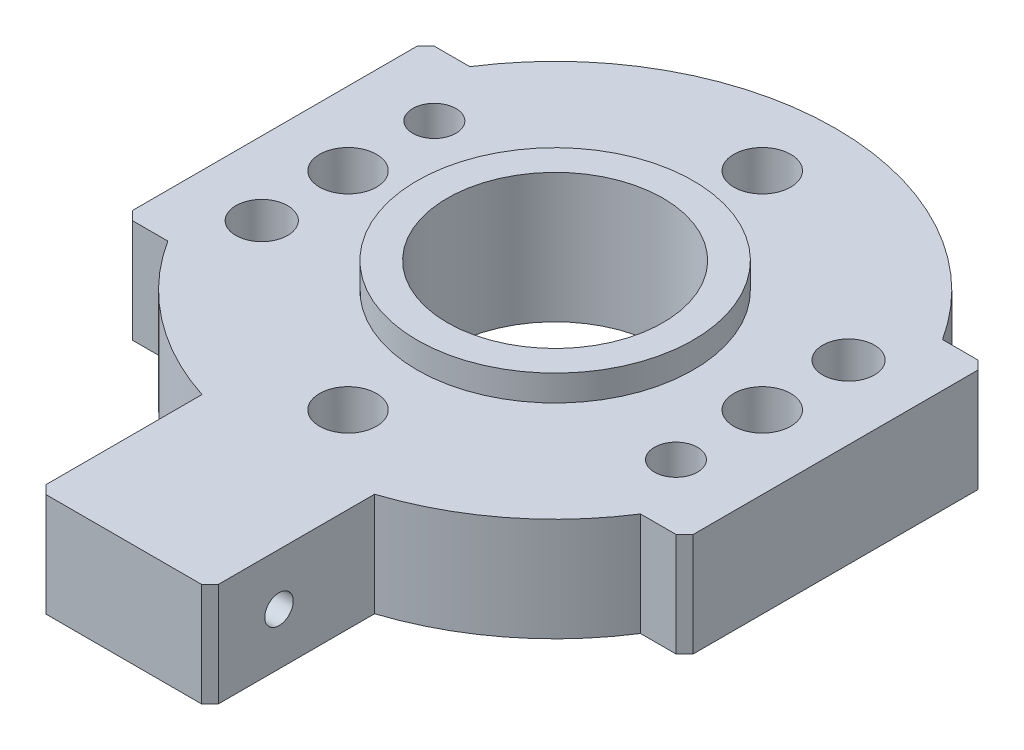
SolidWorks part; units mm, degrees
material "45#"
ref_plane "前基準面" through (0, 0, 0) normal (0, 0, 1) x (1, 0, 0)
ref_plane "上基準面" through (0, 0, 0) normal (0, 1, 0) x (1, 0, 0)
ref_plane "右基準面" through (0, 0, 0) normal (1, 0, 0) x (0, 0, -1)
sketch "草图1" plane through (0, 0, 0) normal (0, 1, 0) x (1, 0, 0)
  line L0 (0, 0) -> (0, -56.3114) construction
  line L1 (-10, -30.9233) -> (-10, -50)
  line L2 (-10, -50) -> (10, -50)
  line L3 (10, -50) -> (10, -30.9233)
  line L4 (0, 0) -> (-41.9616, 0) construction
  line L5 (-32.5, 17.5) -> (-32.5, -17.5)
  line L6 (32.5, 17.5) -> (32.5, -17.5)
  line L7 (-32.5, 17.5) -> (-27.3861, 17.5)
  line L8 (-32.5, -17.5) -> (-27.3861, -17.5)
  line L9 (27.3861, 17.5) -> (32.5, 17.5)
  line L10 (27.3861, -17.5) -> (32.5, -17.5)
  arc A0 (10, -30.9233) -> (27.3861, -17.5) centre (0, 0) ccw
  arc A1 (-27.3861, -17.5) -> (-10, -30.9233) centre (0, 0) ccw
  arc A2 (27.3861, 17.5) -> (-27.3861, 17.5) centre (0, 0) ccw
  dimension "D1" = 65
  dimension "D2" = 20
  dimension "D3" = 50
  dimension "D4" = 35
  dimension "D5" = 65
extrude "凸台-拉伸1" add sketch "草图1" along normal blind 15
sketch "草图2" plane through (0, 15, 0) normal (0, 1, 0) x (1, 0, 0)
  circle A0 centre (0, 0) radius 16
  dimension "D1" = 32
extrude "切除-拉伸1" cut sketch "草图2" against normal blind 3 flip side to cut
sketch "草图3" plane through (0, 0, 0) normal (0, -1, 0) x (1, 0, 0)
  circle A0 centre (0, 0) radius 12.5
  dimension "D1" = 25
extrude "切除-拉伸2" cut sketch "草图3" against normal through all
hole_wizard "M6 六角圆柱头螺钉的柱形沉头孔1" positions "草图4" profile "草图5" counterbore size "M6" standard "GB" end condition up to next
sketch "草图4" plane through (0, 0, 0) normal (0, -1, 0) x (-1, 0, 0)
  line L0 (0, 0) -> (41.7347, 0) construction
  circle A0 centre (0, 0) radius 24 construction
  point P0 (0, 24)
  point P12 (24, 0)
  point P13 (0, -24)
  point P14 (-24, 0)
  dimension "D1" = 48
  dimension "D2" = 4
sketch "草图5" plane through (0, 0, -24) normal (1, 0, 0) x (0, 0, -1)
  line L0 (0, 0) -> (0, 12)
  line L1 (0, 12) -> (3.3, 12)
  line L3 (3.3, 12) -> (3.3, 6.8)
  line L4 (3.3, 6.8) -> (5, 6.8)
  line L5 (5, 6.8) -> (5, 0)
  line L7 (5, 0) -> (0, 0)
  line L11 (0, -6.35) -> (0, 107.95) construction
  dimension "通孔孔直径" = 6.6
  dimension "通孔孔深度" = 12
  dimension "柱形沉头孔直径" = 10
  dimension "柱形沉头孔深度" = 6.8
hole_wizard "Ø6.0mm 暗销孔1" positions "草图6" profile "草图7" hole size "Ø6.0" standard "GB" end condition up to next
sketch "草图6" plane through (0, 0, 0) normal (0, -1, 0) x (-1, 0, 0)
  line L3 (0, 0) -> (-37.4835, 0) construction
  line L4 (24, 10) -> (24, -10) construction
  line L5 (24, -10) -> (-24, -10) construction
  line L6 (-24, -10) -> (-24, 10) construction
  line L7 (-24, 10) -> (24, 10) construction
  line L8 (0, 0) -> (0, -54.5452) construction
  point P110 (24, -10)
  point P119 (-24, 10)
  point P128 (-24, 10)
  dimension "D1" = 20
  dimension "D2" = 48
sketch "草图7" plane through (24, 0, -10) normal (1, 0, 0) x (0, 0, -1)
  line L0 (0, 0) -> (0, 12)
  line L1 (0, 12) -> (3, 12)
  line L2 (3, 12) -> (3, 0)
  line L5 (3, 0) -> (0, 0)
  line L11 (0, -6.35) -> (0, 107.95) construction
  dimension "通孔孔直径" = 6
  dimension "通孔孔深度" = 12
hole_wizard "M4 螺纹孔1" positions "草图8" profile "草图9" tap size "M4" standard "GB" end condition up to next
sketch "草图8" plane through (-10, 0, 0) normal (-1, 0, 0) x (0, 0, 1)
  line L0 (50, 6) -> (21.5605, 6) construction
  line L1 (50, 12) -> (50, 0) construction
  point P0 (42, 6)
  dimension "D1" = 8
sketch "草图9" plane through (-10, 6, 42) normal (0, 1, 0) x (0, 0, 1)
  line L0 (0, 0) -> (0, 20)
  line L1 (0, 20) -> (1.65, 20)
  line L2 (1.65, 20) -> (1.65, 0)
  line L5 (1.65, 0) -> (0, 0)
  line L11 (0, -6.35) -> (0, 107.95) construction
  dimension "通孔螺纹孔钻头直径" = 3.3
  dimension "通孔螺纹孔钻头深度" = 20
cosmetic thread "孔螺蚊线1" parameters "D2"=4
hole_wizard "M6 螺纹孔2" positions "草图10" profile "草图11" tap size "M6" standard "GB" end condition up to next
sketch "草图10" plane through (0, 0, 0) normal (0, -1, 0) x (-1, 0, 0)
  line L0 (24, -10) -> (-24, -10) construction
  line L1 (-24, -10) -> (-24, 10) construction
  line L2 (-24, 10) -> (24, 10) construction
  line L3 (24, 10) -> (24, -10) construction
  point P36 (24, 10)
  point P41 (-24, -10)
  point P56 (-24, -10)
sketch "草图11" plane through (-24, 0, -10) normal (1, 0, 0) x (0, 0, -1)
  line L0 (0, 0) -> (0, 12)
  line L1 (0, 12) -> (2.5, 12)
  line L2 (2.5, 12) -> (2.5, 0)
  line L5 (2.5, 0) -> (0, 0)
  line L11 (0, -6.35) -> (0, 107.95) construction
  dimension "通孔螺纹孔钻头直径" = 5
  dimension "通孔螺纹孔钻头深度" = 12
cosmetic thread "孔螺蚊线2" parameters "D2"=6
cosmetic thread "孔螺蚊线6" parameters "D2"=6
chamfer "倒角1" distance 1 angle 45 6 edges at (10, 6, 50) (-10, 6, 50) (32.5, 6, -17.5) (32.5, 6, 17.5) (-32.5, 6, -17.5) (-32.5, 6, 17.5)
